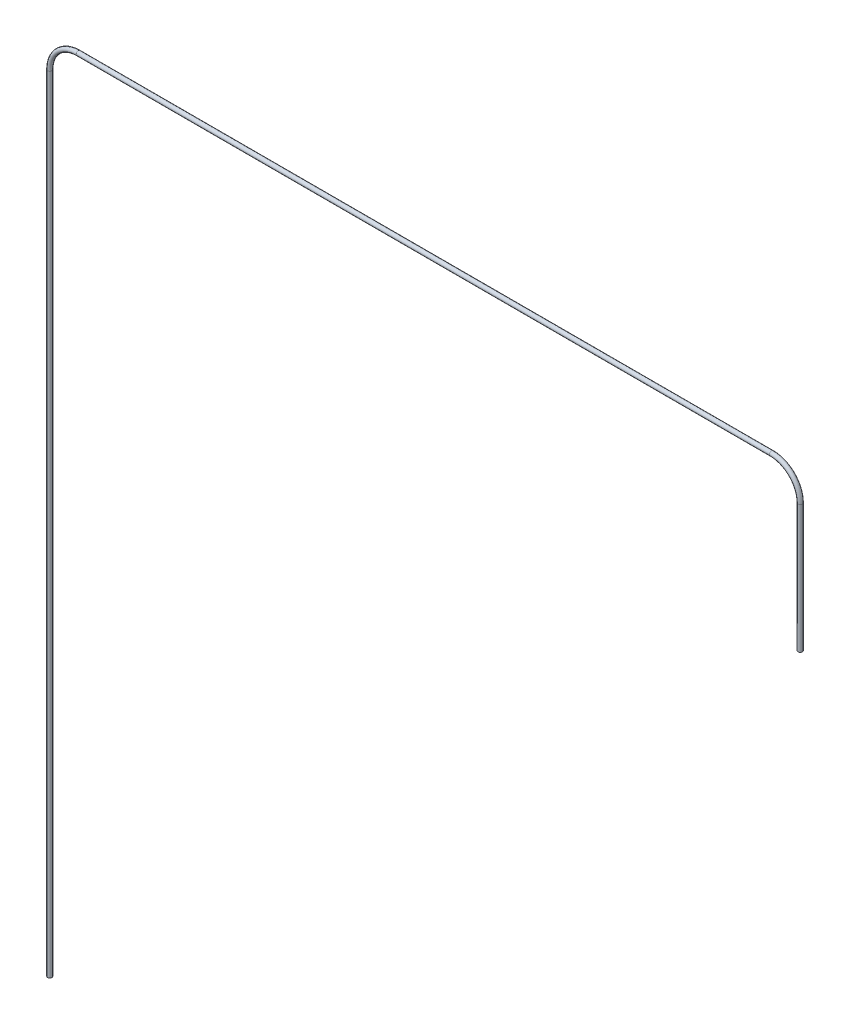
SolidWorks part; units mm, degrees
ref_plane "Front Plane" through (0, 0, 0) normal (0, 0, 1) x (1, 0, 0)
ref_plane "Top Plane" through (0, 0, 0) normal (0, 1, 0) x (1, 0, 0)
ref_plane "Right Plane" through (0, 0, 0) normal (1, 0, 0) x (0, 0, -1)
sketch "Sketch1" plane through (0, 0, 0) normal (0, 0, 1) x (1, 0, 0)
  line L0 (0, 0) -> (0, 1153)
  line L1 (42, 1195) -> (1060, 1195)
  line L2 (1102, 1153) -> (1102, 965)
  arc A0 (1060, 1195) -> (1102, 1153) centre (1060, 1153) cw
  arc A1 (0, 1153) -> (42, 1195) centre (42, 1153) cw
  point P7 (1102, 1195)
  point P10 (0, 1195)
  dimension "D3" = 42
  dimension "D1" = 1102
  dimension "D2" = 1195
  dimension "D4" = 230
sketch "Sketch2" plane through (0, 0, 0) normal (0, 1, 0) x (1, 0, 0)
  circle A0 centre (0, 0) radius 3.25
  dimension "D1" = 6.5
sweep "Sweep1" add profiles "Sketch2" path "Sketch1"
